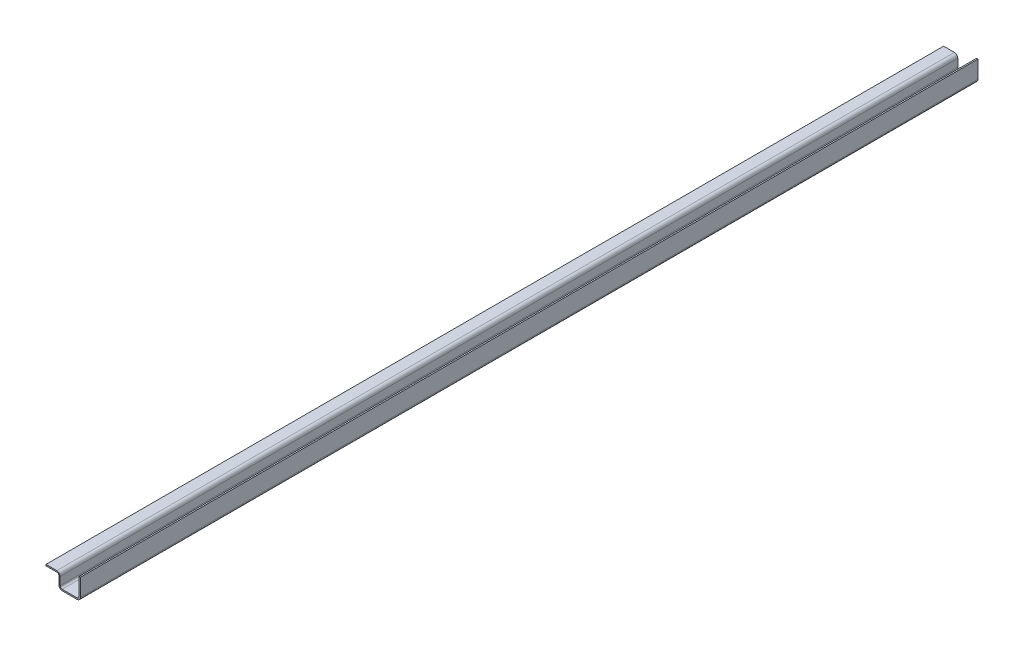
from build123d import *

# Parameters (mm, degrees)
EXTRUDE_1_DEPTH = 665.5


with BuildPart() as part:
    # 草图1 → 拉伸-薄壁1 (new, symmetric)
    with BuildSketch(Plane.XY):
        with BuildLine():
            Line((-1, 30), (-1, 4))
            ThreePointArc((-1, 4), (-1.878679656, 1.878679656), (-4, 1))
            Line((-4, 1), (-26, 1))
            ThreePointArc((-26, 1), (-28.121320344, 1.878679656), (-29, 4))
            Line((-29, 4), (-29, 16))
            ThreePointArc((-29, 16), (-30.464466094, 19.535533906), (-34, 21))
            Line((-34, 21), (-50, 21))
            Line((-50, 21), (-50, 19))
            Line((-50, 19), (-34, 19))
            ThreePointArc((-34, 19), (-31.878679656, 18.121320344), (-31, 16))
            Line((-31, 16), (-31, 4))
            ThreePointArc((-31, 4), (-29.535533906, 0.464466094), (-26, -1))
            Line((-26, -1), (-4, -1))
            ThreePointArc((-4, -1), (-0.464466094, 0.464466094), (1, 4))
            Line((1, 4), (1, 30))
            Line((1, 30), (-1, 30))
        make_face()
    extrude(amount=EXTRUDE_1_DEPTH, both=True)


solid = part.part
